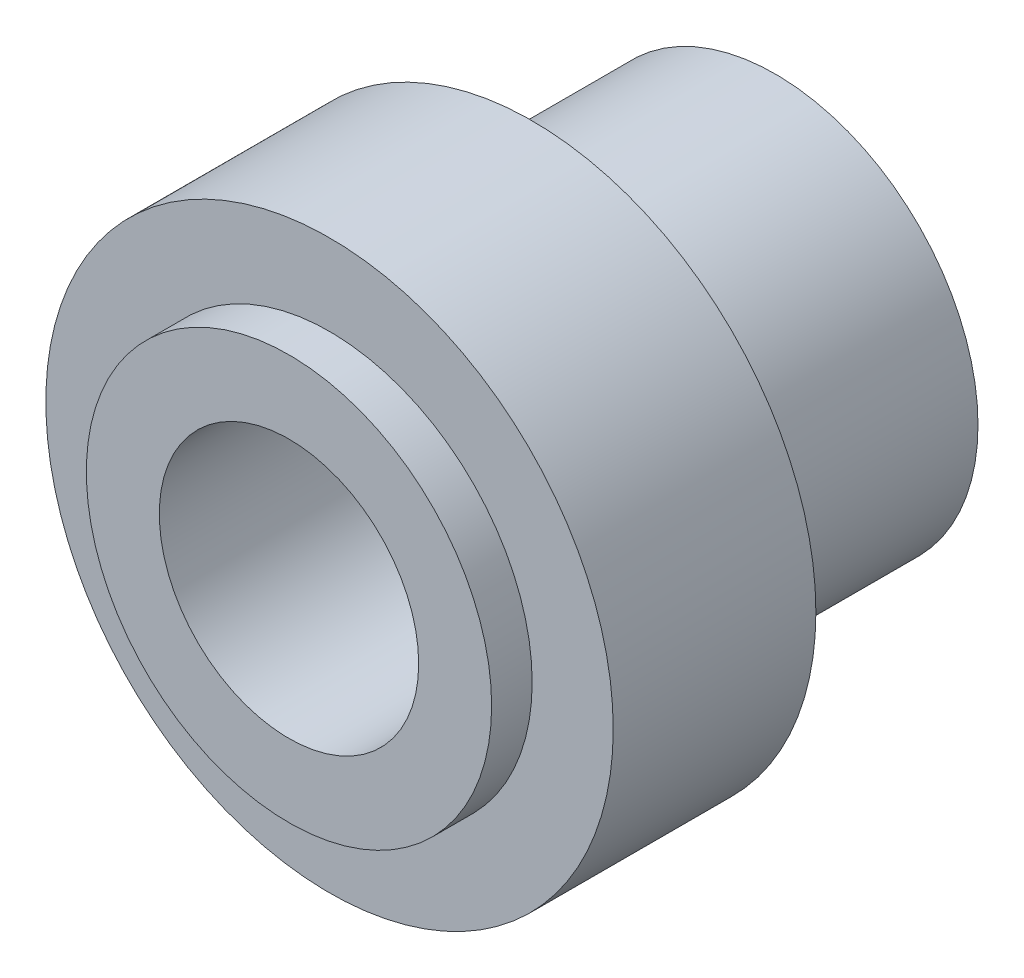
SolidWorks part; units mm, degrees
ref_plane "前视基准面" through (0, 0, 0) normal (0, 0, 1) x (1, 0, 0)
ref_plane "上视基准面" through (0, 0, 0) normal (0, 1, 0) x (1, 0, 0)
ref_plane "右视基准面" through (0, 0, 0) normal (1, 0, 0) x (0, 0, -1)
other "Configuration Table"
sketch "草图1" plane through (0, 0, 0) normal (0, 0, 1) x (1, 0, 0)
  circle A0 centre (0, 0) radius 5
  circle A1 centre (0, 0) radius 3.2
  point P0 (0, 0)
  dimension "D1" = 6.4
  dimension "D2" = 10
extrude "凸台-拉伸1" add sketch "草图1" against normal mid plane 12
sketch "草图2" plane through (0, 0, 0) normal (0, 0, 1) x (1, 0, 0)
  circle A0 centre (0, 0) radius 7
  circle A1 centre (0, 0) radius 3.2
  point P0 (0, 0)
  dimension "D1" = 6.4
  dimension "D2" = 14
extrude "凸台-拉伸2" add sketch "草图2" along normal blind 5
